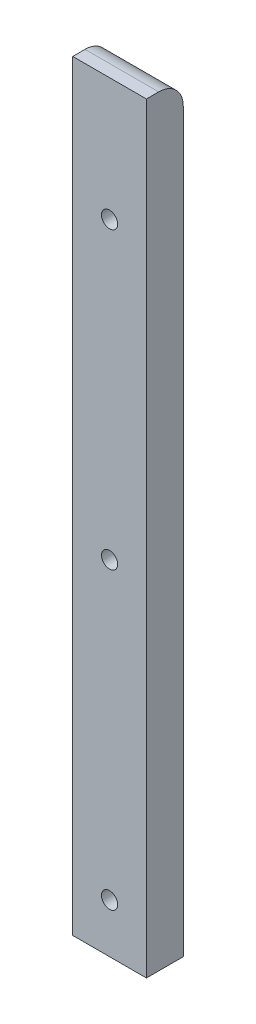
SolidWorks part; units mm, degrees
material "白色POM"
ref_plane "前基準面" through (0, 0, 0) normal (0, 0, 1) x (1, 0, 0)
ref_plane "上基準面" through (0, 0, 0) normal (0, 1, 0) x (1, 0, 0)
ref_plane "右基準面" through (0, 0, 0) normal (1, 0, 0) x (0, 0, -1)
sketch "草图1" plane through (0, 0, 0) normal (0, 0, 1) x (1, 0, 0)
  line L1 (-15, 155) -> (15, 155)
  line L2 (-15, 155) -> (-15, -155)
  line L3 (-15, -155) -> (15, -155)
  line L4 (15, 155) -> (15, -155)
  line L5 (-15, 155) -> (15, -155) construction
  line L6 (-15, -155) -> (15, 155) construction
  point P0 (0, 0)
  dimension "D1" = 30
  dimension "D2" = 310
extrude "凸台-拉伸1" add sketch "草图1" along normal blind 15
hole_wizard "打孔尺寸(%根据)内六角圆柱头螺钉的类型1" positions "草图3" profile "草图2" counterbore size "M6" standard "GB" end condition through all
sketch "草图3" plane through (0, 0, 0) normal (0, 0, -1) x (-1, 0, 0)
  line L0 (0, 155) -> (0, 105) construction
  line L1 (-15, 155) -> (15, 155) construction
  point P0 (0, 105)
  point P2 (0, -15)
  point P4 (0, -135)
  dimension "D1" = 50
  dimension "D2" = 120
  dimension "D3" = 120
sketch "草图2" plane through (0, 105, 0) normal (1, 0, 0) x (0, 1, 0)
  line L0 (0, 0) -> (0, 15)
  line L1 (0, 15) -> (3.3, 15)
  line L3 (3.3, 15) -> (3.3, 6.8)
  line L4 (3.3, 6.8) -> (5.5, 6.8)
  line L5 (5.5, 6.8) -> (5.5, 0)
  line L7 (5.5, 0) -> (0, 0)
  line L11 (0, -6.35) -> (0, 107.95) construction
  dimension "通孔孔直径" = 6.6
  dimension "通孔孔深度" = 15
  dimension "柱形沉头孔直径" = 11
  dimension "柱形沉头孔深度" = 6.8
fillet "圆角1" radius 10 1 edges at (0, 155, 0)
